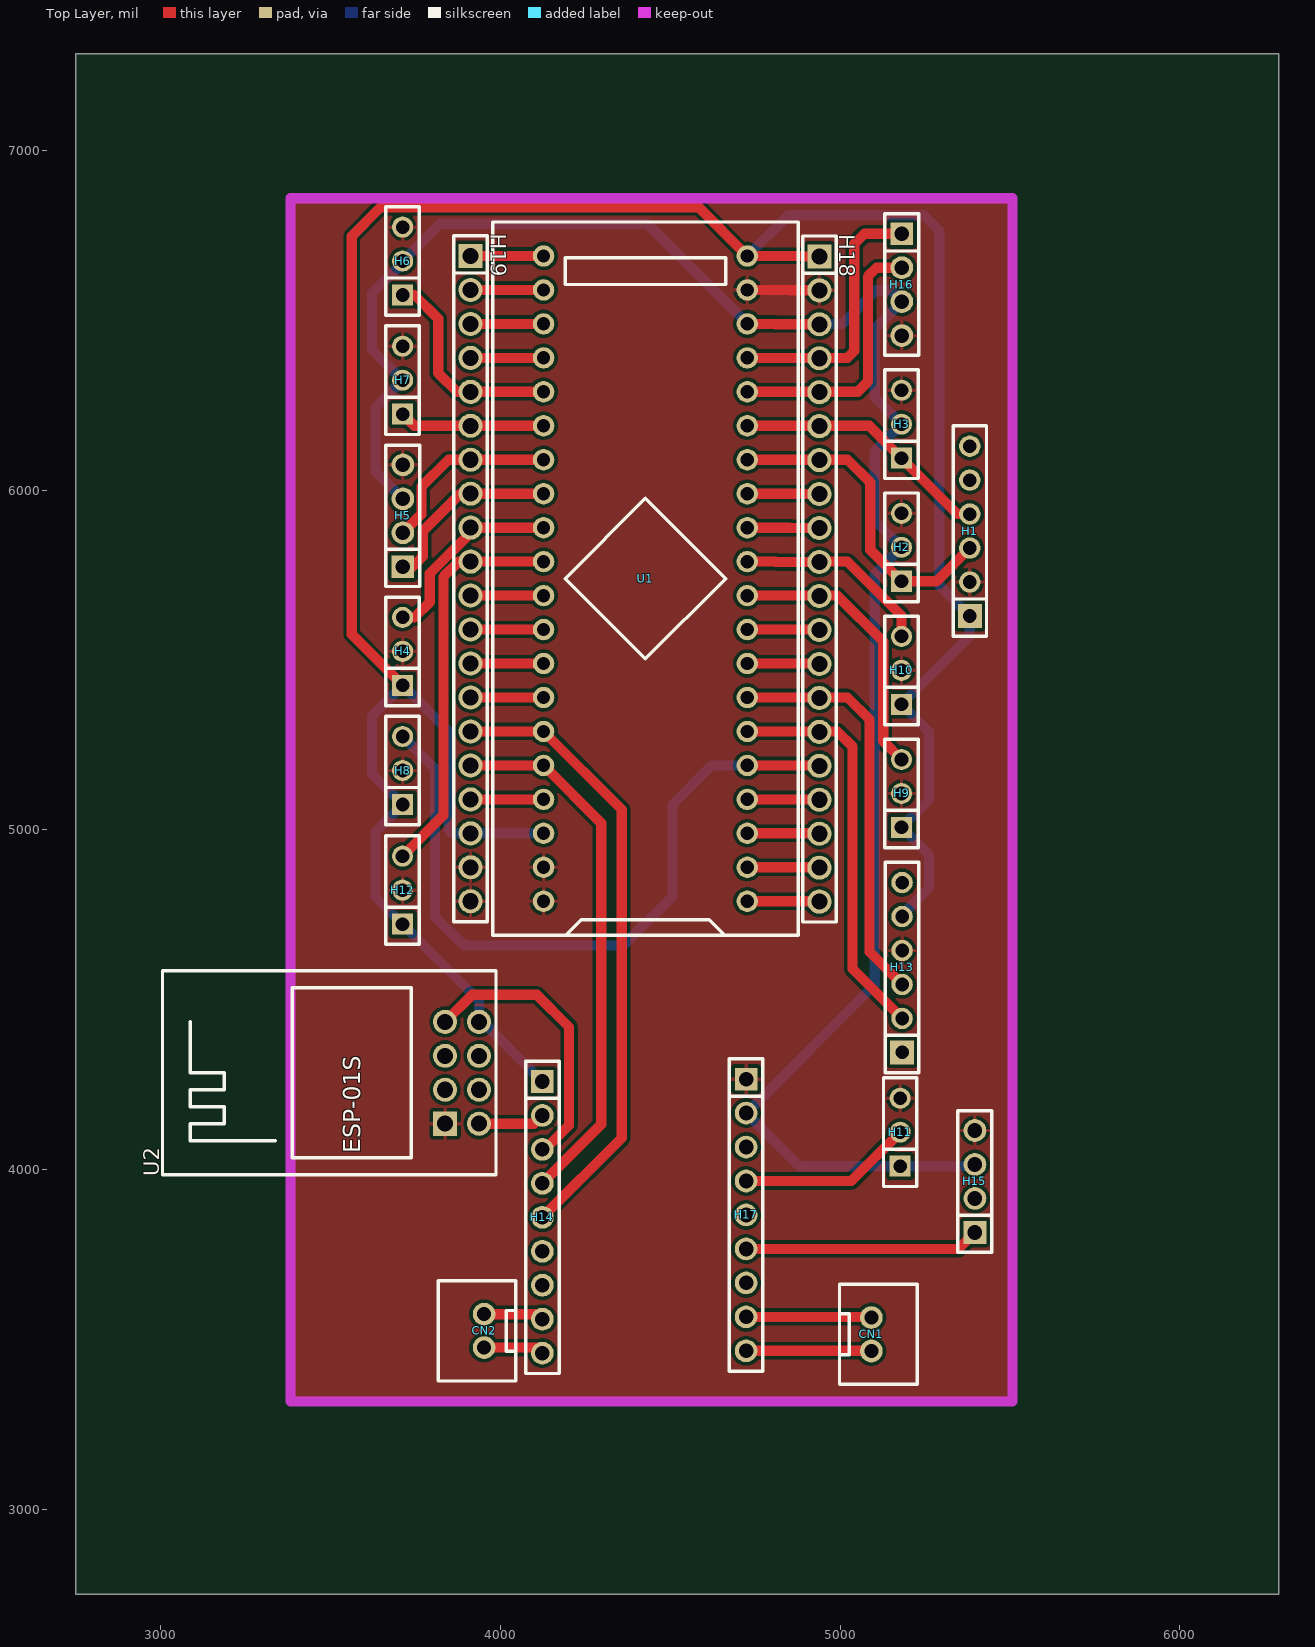
[diagram p0: Top Layer view]
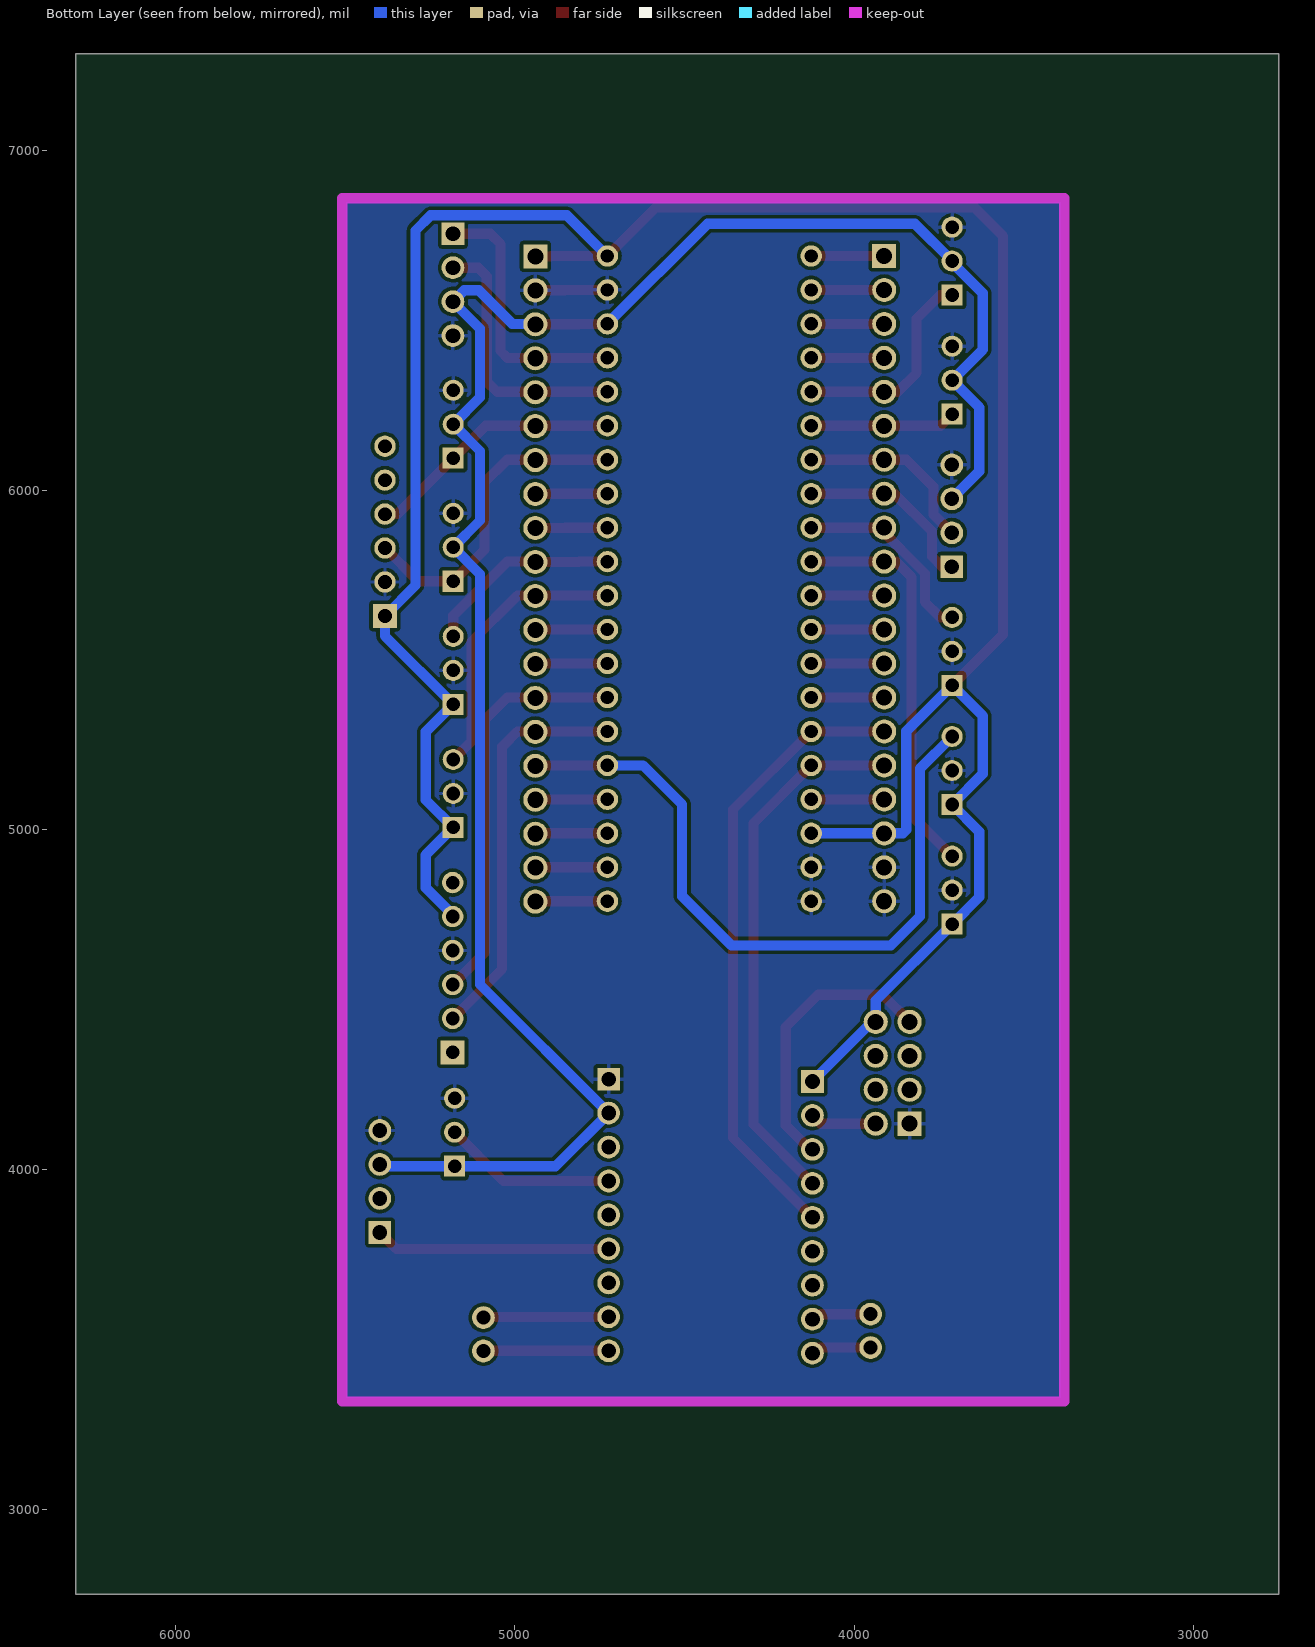
[diagram p1: Bottom Layer view, seen from below]
# Altium PCB MISC51613.pcbdoc
Units mil, origin at the board's own origin, x right, y up, seen from the top; angles counter-clockwise.
Board outline 3542 x 4535 mil, 2 copper layers (Top Layer, Bottom Layer), stack 62.206 mil thick; 23 components, 45 nets, 164 pads, 0 vias.

## Layer stack, top to bottom
Top Solder Mask Layer: solder mask 0.394, Dk 3.3
Top Layer: signal copper 1.379
Dielectric1: surface 59.449, FR4, Dk 4.5
Bottom Layer: signal copper 1.378
Bottom Solder Mask Layer: solder mask 0.394, Dk 3.3

## Board outline
6292,2750 2750,2750 2750,7285 6292,7285

## Design rules (kind name [scope] priority, off if disabled: settings)
BoardOutlineClearance copperThickness2oz_1 [All] p2 off: genericclearance=7.99 ignorepadtopadclearanceinfootprint=FALSE except(0: Arc-SplitContinuation Track-SplitContinuation SMDPad-SplitContinuation THPad-SplitContinuation Via-SplitContinuation Fill-SplitContinuation Region-SplitContinuation Poly-SplitContinuation Text-SplitContinuation Hole-SplitContinuation; 5.98: Arc-CutoutEdge Track-CutoutEdge SMDPad-CutoutEdge THPad-CutoutEdge Via-CutoutEdge Text-CutoutEdge; 6.9: Hole-OutlineEdge Hole-CutoutEdge; 10: Poly-OutlineEdge Poly-CutoutEdge; 11.81: Arc-OutlineEdge Track-OutlineEdge SMDPad-OutlineEdge THPad-OutlineEdge Via-OutlineEdge Fill-OutlineEdge Region-OutlineEdge Text-OutlineEdge Fill-CutoutEdge Region-CutoutEdge)
BoardOutlineClearance Plane_innerPlane_1 [All] p4 off: genericclearance=4.02 ignorepadtopadclearanceinfootprint=FALSE except(0: Arc-SplitContinuation Track-SplitContinuation SMDPad-SplitContinuation THPad-SplitContinuation Via-SplitContinuation Fill-SplitContinuation Region-SplitContinuation Poly-SplitContinuation Text-SplitContinuation Hole-SplitContinuation; 5.98: Arc-CutoutEdge Track-CutoutEdge SMDPad-CutoutEdge THPad-CutoutEdge Via-CutoutEdge Text-CutoutEdge; 6.9: Hole-OutlineEdge Hole-CutoutEdge; 10: Poly-OutlineEdge Poly-CutoutEdge; 11.81: Arc-OutlineEdge Track-OutlineEdge SMDPad-OutlineEdge THPad-OutlineEdge Via-OutlineEdge Fill-OutlineEdge Region-OutlineEdge Text-OutlineEdge Fill-CutoutEdge Region-CutoutEdge)
BoardOutlineClearance Copper_copperRegion_1 [All] p6 off: genericclearance=4.02 ignorepadtopadclearanceinfootprint=FALSE except(0: Arc-SplitContinuation Track-SplitContinuation SMDPad-SplitContinuation THPad-SplitContinuation Via-SplitContinuation Fill-SplitContinuation Region-SplitContinuation Poly-SplitContinuation Text-SplitContinuation Hole-SplitContinuation; 5.98: Arc-CutoutEdge Track-CutoutEdge SMDPad-CutoutEdge THPad-CutoutEdge Via-CutoutEdge Text-CutoutEdge; 6.9: Hole-OutlineEdge Hole-CutoutEdge; 10: Poly-OutlineEdge Poly-CutoutEdge; 11.81: Arc-OutlineEdge Track-OutlineEdge SMDPad-OutlineEdge THPad-OutlineEdge Via-OutlineEdge Fill-OutlineEdge Region-OutlineEdge Text-OutlineEdge Fill-CutoutEdge Region-CutoutEdge)
BoardOutlineClearance copperThickness1oz_1 [All] p8: genericclearance=4.02 ignorepadtopadclearanceinfootprint=FALSE except(0: Arc-SplitContinuation Track-SplitContinuation SMDPad-SplitContinuation THPad-SplitContinuation Via-SplitContinuation Fill-SplitContinuation Region-SplitContinuation Poly-SplitContinuation Text-SplitContinuation Hole-SplitContinuation; 5.98: Arc-CutoutEdge Track-CutoutEdge SMDPad-CutoutEdge THPad-CutoutEdge Via-CutoutEdge Text-CutoutEdge; 6.9: Hole-OutlineEdge Hole-CutoutEdge; 10: Poly-OutlineEdge Poly-CutoutEdge; 11.81: Arc-OutlineEdge Track-OutlineEdge SMDPad-OutlineEdge THPad-OutlineEdge Via-OutlineEdge Fill-OutlineEdge Region-OutlineEdge Text-OutlineEdge Fill-CutoutEdge Region-CutoutEdge)
Clearance copperThickness2oz [All] p1 off: gap=7.99 ignorepadtopadclearanceinfootprint=FALSE except(5.98: SMDPad-Track SMDPad-SMDPad THPad-Track SMDPad-THPad THPad-THPad Track-Via SMDPad-Via THPad-Via Via-Via Fill-SMDPad Region-SMDPad Fill-THPad Region-THPad Fill-Via Region-Via Fill-Fill Fill-Region Region-Region Arc-Track Arc-SMDPad Arc-THPad Arc-Via Fill-Arc Region-Arc Arc-Arc Text-Track SMDPad-Text Text-THPad Text-Via Fill-Text Region-Text Arc-Text Text-Text; 6.9: Hole-Track Hole-SMDPad Hole-THPad Hole-Via Fill-Hole Region-Hole Hole-Arc Hole-Text; 10: Poly-Track Poly-SMDPad Poly-THPad Poly-Via Poly-Fill Poly-Region Poly-Poly Poly-Arc Poly-Text Poly-Hole; 11.81: Fill-Track Region-Track)
Clearance Plane_innerPlane [All] p3 off: gap=4.02 ignorepadtopadclearanceinfootprint=FALSE except(5.98: SMDPad-Track SMDPad-SMDPad THPad-Track SMDPad-THPad THPad-THPad Track-Via SMDPad-Via THPad-Via Via-Via Fill-SMDPad Region-SMDPad Fill-THPad Region-THPad Fill-Via Region-Via Fill-Fill Fill-Region Region-Region Arc-Track Arc-SMDPad Arc-THPad Arc-Via Fill-Arc Region-Arc Arc-Arc Text-Track SMDPad-Text Text-THPad Text-Via Fill-Text Region-Text Arc-Text Text-Text; 6.9: Hole-Track Hole-SMDPad Hole-THPad Hole-Via Fill-Hole Region-Hole Hole-Arc Hole-Text; 10: Poly-Track Poly-SMDPad Poly-THPad Poly-Via Poly-Fill Poly-Region Poly-Poly Poly-Arc Poly-Text Poly-Hole; 11.81: Fill-Track Region-Track)
Clearance Copper_copperRegion [All] p5 off: gap=4.02 ignorepadtopadclearanceinfootprint=FALSE except(5.98: SMDPad-Track SMDPad-SMDPad THPad-Track SMDPad-THPad THPad-THPad Track-Via SMDPad-Via THPad-Via Via-Via Fill-SMDPad Region-SMDPad Fill-THPad Region-THPad Fill-Via Region-Via Fill-Fill Fill-Region Region-Region Arc-Track Arc-SMDPad Arc-THPad Arc-Via Fill-Arc Region-Arc Arc-Arc Text-Track SMDPad-Text Text-THPad Text-Via Fill-Text Region-Text Arc-Text Text-Text; 6.9: Hole-Track Hole-SMDPad Hole-THPad Hole-Via Fill-Hole Region-Hole Hole-Arc Hole-Text; 10: Poly-Track Poly-SMDPad Poly-THPad Poly-Via Poly-Fill Poly-Region Poly-Poly Poly-Arc Poly-Text Poly-Hole; 11.81: Fill-Track Region-Track)
Clearance copperThickness1oz [All] p7: gap=4.02 ignorepadtopadclearanceinfootprint=FALSE except(5.98: SMDPad-Track SMDPad-SMDPad THPad-Track SMDPad-THPad THPad-THPad Track-Via SMDPad-Via THPad-Via Via-Via Fill-SMDPad Region-SMDPad Fill-THPad Region-THPad Fill-Via Region-Via Fill-Fill Fill-Region Region-Region Arc-Track Arc-SMDPad Arc-THPad Arc-Via Fill-Arc Region-Arc Arc-Arc Text-Track SMDPad-Text Text-THPad Text-Via Fill-Text Region-Text Arc-Text Text-Text; 6.9: Hole-Track Hole-SMDPad Hole-THPad Hole-Via Fill-Hole Region-Hole Hole-Arc Hole-Text; 10: Poly-Track Poly-SMDPad Poly-THPad Poly-Via Poly-Fill Poly-Region Poly-Poly Poly-Arc Poly-Text Poly-Hole; 11.81: Fill-Track Region-Track)
DiffPairsRouting differentialPair [All] p1: maxlimit=6 minlimit=6 mostfreqgap=6 toplayer_minwidth=5 toplayer_prefwidth=10 toplayer_maxwidth=100 toplayer_mingap=6 toplayer_prefgap=6 toplayer_maxgap=6 bottomlayer_minwidth=5 bottomlayer_prefwidth=10 bottomlayer_maxwidth=100 bottomlayer_mingap=6 bottomlayer_prefgap=6 bottomlayer_maxgap=6 maxuncoupledlength=10
HoleToHoleClearance otherClearance [All] p1: gap=11.81 allowstackedmicrovias=TRUE
Length netLength [All] p1: minlimit=0 maxlimit=0
PasteMaskExpansion pasteMaskExpansion [All] p1: expansion=0
PlaneConnect innerPlane [All] p1: planeconnectstyle=Relief reliefexpansion=20 reliefentries=4 reliefconductorwidth=10 reliefairgap=10
PolygonConnect copperRegion [(InNet('GND'))] p1: connectstyle=Relief reliefconductorwidth=10 reliefentries=4 polygonreliefangle="90 Angle" airgapwidth=10 via.connectstyle=Relief via.reliefconductorwidth=10 via.reliefentries=4 via.polygonreliefangle="90 Angle" via.airgapwidth=10
RoutingVias viaSize [All] p1: holewidth=12.01 width=24.02 viastyle="Through Hole" minholewidth=11.81 minwidth=19.68 maxholewidth=248.03 maxwidth=393.7
SolderMaskExpansion solderMaskExpansion [IsVia] p1: expansion=-1000 istentingtop=TRUE
SolderMaskExpansion solderMaskExpansion [All] p2: expansion=2 istentingtop=FALSE
Width copperThickness2oz_2 [All] p1 off: maxlimit=100 minlimit=8 preferedwidth=10
Width copperThickness1oz_2 [All] p2: maxlimit=100 minlimit=5 preferedwidth=10

## Components (designator, comment, footprint, x,y, rotation, side; value= is the part's Value field where it differs from the comment)
CN1 "XH2.54*2P_through-hole" CONN-TH_2P-P2.50-XH2.54-2P 5092,3515 r90 top
CN2 "XH2.54*2P_through-hole" CONN-TH_2P-P2.50-XH2.54-2P 3952,3525 r270 top
H1 "" HDR-TH_6P-P2.54-V-F 5382,5880 r90 top
H2 "" HDR-TH_3P-P2.54-V-F 5181.06,5832.25 r90 top
H3 "" HDR-TH_3P-P2.54-V-F 5181.06,6194.66 r90 top
H4 "" HDR-TH_3P-P2.54-V-F 3712,5525.79 r90 top
H5 "" HDR-TH_4P-P2.54-V-F 3712.79,5925 r90 top
H6 "" HDR-TH_3P-P2.54-V-F 3712,6675 r90 top
H7 "" HDR-TH_3P-P2.54-V-F 3712,6324.21 r90 top
H8 "" HDR-TH_3P-P2.54-V-F 3712,5175 r90 top
H9 "" HDR-TH_3P-P2.54-V-F 5181.06,5107.42 r90 top
H10 "" HDR-TH_3P-P2.54-V-F 5181.06,5469.83 r90 top
H11 "" HDR-TH_3P-P2.54-V-F 5177,4110 r90 top
H12 "" HDR-TH_3P-P2.54-V-F 3711.84,4822.79 r90 top
H13 "" HDR-TH_6P-P2.54-V-F 5182.63,4595 r90 top
H14 "" HDR-TH_9P-P2.54-V-F-1 4123.42,3859.44 r270 top
H15 "" HDR-TH_4P-P2.54-V-F 5397,3965 r90 top
H16 "" HDR-TH_4P-P2.54-V-F 5181.84,6605.51 r270 top
H17 "" HDR-TH_9P-P2.54-V-F-1 4723.42,3866.33 r270 top
H18 "" HDR-TH_20P-P2.54-V-F 4939.11,5738.84 r270 top
H19 "" HDR-TH_20P-P2.54-V-F 3912,5740 r270 top
U1 "STM32F103C8T6-Card" CONN-TH_L53.3-W22.9_STM32F103C8T6-CARD 4427,5740 r90 top
U2 "ESP-01S" WIFIM-TH_ESP-01S 3887,4285 r90 top

## Footprints (in the part's own frame and the unit in brackets; to place one, negate y for a bottom-side part, rotate by r counter-clockwise, add the part's x,y. Pads: shape width x height; smd on the part's side, far side on the other; paste and mask are expansions set on the pad)
CONN-TH_2P-P2.50-XH2.54-2P [mm]
  round 1.7 hole 1.05 paste+0 mask+0.05: 1(1.25,0) 2(-1.25,0)
  silkscreen extent -3.75,-3.42 3.75,2.37
CONN-TH_L53.3-W22.9_STM32F103C8T6-CARD [mm]
  round 1.6 hole 1: 1(-24.13,-7.62) 2(-21.59,-7.62) 3(-19.05,-7.62) 4(-16.51,-7.62) 5(-13.97,-7.62) 6(-11.43,-7.62) 7(-8.89,-7.62) 8(-6.35,-7.62) 9(-3.81,-7.62) 10(-1.27,-7.62) 11(1.27,-7.62) 12(3.81,-7.62) 13(6.35,-7.62) 14(8.89,-7.62) 15(11.43,-7.62) 16(13.97,-7.62) 17(16.51,-7.62) 18(19.05,-7.62) 19(21.59,-7.62) 20(24.13,-7.62) 21(24.13,7.62) 22(21.59,7.62) 23(19.05,7.62) 24(16.51,7.62) 25(13.97,7.62) 26(11.43,7.62) 27(8.89,7.62) 28(6.35,7.62) 29(3.81,7.62) 30(1.27,7.62) 31(-1.27,7.62) 32(-3.81,7.62) 33(-6.35,7.62) 34(-8.89,7.62) 35(-11.43,7.62) 36(-13.97,7.62) 37(-16.51,7.62) 38(-19.05,7.62) 39(-21.59,7.62) 40(-24.13,7.62)
  silkscreen extent -26.67,-11.43 26.67,11.43
HDR-TH_3P-P2.54-V-F [mil]
  rect 62x62 hole 40.16: 1(-100,0)
  round 62 hole 40.16: 2(0,0) 3(100,0)
  silkscreen extent -160,-49 160,49
HDR-TH_4P-P2.54-V-F [mm]
  rect 1.7x1.7 hole 1.1: 1(-3.81,0)
  round 1.7 hole 1.1: 2(-1.27,0) 3(1.27,0) 4(3.81,0)
  silkscreen extent -5.29,-1.27 5.29,1.27
HDR-TH_6P-P2.54-V-F [mm]
  rect 1.8x1.8 hole 1.02: 1(-6.35,0)
  round 1.6 hole 1.02: 2(-3.81,0) 3(-1.27,0) 4(1.27,0) 5(3.81,0) 6(6.35,0)
  silkscreen extent -7.87,-1.25 7.87,1.25
HDR-TH_9P-P2.54-V-F-1 [mm]
  rect 1.7x1.7 hole 1.1: 1(-10.16,0)
  round 1.7 hole 1.1: 2(-7.62,0) 3(-5.08,0) 4(-2.54,0) 5(0,0) 6(2.54,0) 7(5.08,0) 8(7.62,0) 9(10.16,0)
  silkscreen extent -11.68,-1.25 11.68,1.25
HDR-TH_20P-P2.54-V-F [mm]
  rect 1.8x1.8 hole 1.2: 1(-24.13,0)
  round 1.8 hole 1.2: 2(-21.59,0) 3(-19.05,0) 4(-16.51,0) 5(-13.97,0) 6(-11.43,0) 7(-8.89,0) 8(-6.35,0) 9(-3.81,0) 10(-1.27,0) 11(1.27,0) 12(3.81,0) 13(6.35,0) 14(8.89,0) 15(11.43,0) 16(13.97,0) 17(16.51,0) 18(19.05,0) 19(21.59,0) 20(24.13,0)
  silkscreen extent -25.65,-1.25 25.65,1.25
WIFIM-TH_ESP-01S [mm]
  rect 1.8x1.8 hole 1.2: 1(-3.81,1.27)
  round 1.8 hole 1.2: 2(-1.27,1.27) 3(1.27,1.27) 4(3.81,1.27) 5(3.81,-1.27) 6(1.27,-1.27) 7(-1.27,-1.27) 8(-3.81,-1.27)
  silkscreen extent -7.62,-2.54 7.62,22.4

## Nets (pads, with @x,y where several pads share a name; then routed paths per layer and width w, separated by ;. In a path a pad name is that pad's centre, name@x,y a point inside that pad or via, vN(x,y) a via of type N, cw(c..) or ccw(c..) an arc to the next point about the centre after c; other vN are vias at no path point)
$1N17166: H15.1 H17.6 | length 693.7
  Top Layer w30: H17.6 5348.33,3766.33 H15.1
$1N17173: H11.2 H17.4 | length 513.1
  Top Layer w30: H17.4 5033.33,3966.33 H11.2
+5V: H2.2 H3.2 H5.3 H6.2 H7.2 H11.1 H15.3 H16.3 H17.2 H18.3 U1.18 | length 5984.5
  Top Layer w30: U1.18 4809.67,6490 4810.83,6488.84 H18.3
  Bottom Layer w30: H5.3 3632,6055.79 3632,6244.21 H7.2 3622,6414.21 3622,6580 3712,6670 H6.2 3822,6785 4432,6785 U1.18 ; H18.3@4939.11,6490 5007,6490 5105.96,6588.96 5148.39,6588.96 H16.3 5102,6475.66 5102,6273.72 H3.2 5102,6115.61 5102,5911.3 H2.2 5102,5753.19 5102,4544.92 H17.2 4879.75,4010 H11.1 5392,4010 H15.3
GND: H1.2 H2.3 H3.3 H4.2 H5.4 H6.3 H7.3 H8.2 H9.2 H10.2 H11.3 H12.2 H13.4 H15.4 H16.4 H17.1 H18.2 H19.19 H19.20 U1.19 U1.39 U1.40 U2.1 | length 212.6
  Top Layer w30: U1.19 4851.09,6590 4852.25,6588.84 H18.2
MIC+: CN1.1 H17.8 | length 369.5
  Top Layer w30: H17.8 5089.88,3566.33 CN1.1
MIC-: CN1.2 H17.9 | length 368.8
  Top Layer w30: H17.9 5091.45,3466.33 CN1.2
NRST: H19.17 U1.37 | length 215
  Top Layer w30: H19.17 U1.37
PA0: H6.1 H19.5 U1.25 | length 626.8
  Top Layer w30: H6.1 3747,6575 3817,6505 3817,6345 3872,6290 H19.5 U1.25
PA1: H7.1 H19.6 U1.26 | length 429.2
  Top Layer w30: H7.1 3746.21,6190 H19.6 U1.26
PA2: H5.2 H19.7 U1.27 | length 550.6
  Top Layer w30: H5.2 3767.24,5929.45 3767.24,6010.24 3847,6090 H19.7 U1.27
PA3: H5.1 H19.8 U1.28 | length 546.8
  Top Layer w30: H5.1 3741.25,5775 3771.25,5805 3771.25,5879.25 3882,5990 U1.28
PA4: H4.3 H19.9 U1.29 | length 573.8
  Top Layer w30: H4.3 3747,5625.79 3792,5670.79 3792,5755 3927,5890 U1.29
PA5: H12.3 H19.10 U1.30 | length 1185.6
  Top Layer w30: H12.3 3832,5042.94 3832,5745 3877,5790 U1.30
PA6: H19.11 U1.31 | length 215
  Top Layer w30: H19.11 U1.31
PA7: H19.12 U1.32 | length 215
  Top Layer w30: H19.12 U1.32
PA8: H8.3 H18.16 U1.5 | length 2114.8
  Top Layer w30: U1.5 4937.94,5190 H18.16
  Bottom Layer w30: H8.3 3807,5180 3807,4745 3892,4660 4362,4660 4507,4805 4507,5075 4622,5190 U1.5
PA9: H13.2 H18.15 U1.6 | length 1189
  Top Layer w30: U1.6 4992,5290 5037,5245 5037,4590.63 H13.2
PA10: H13.3 H18.14 U1.7 | length 1206.5
  Top Layer w30: U1.7 5022,5390 5087,5325 5087,4640.63 H13.3
PA11: H18.13 U1.8 | length 212.6
  Top Layer w30: U1.8 4937.94,5490 H18.13
PA12: H18.12 U1.9 | length 212.6
  Top Layer w30: U1.9 4937.94,5590 H18.12
PA15: H9.3 H18.11 U1.10 | length 827.5
  Top Layer w30: U1.10 H18.11@4937.94,5690 ; H18.11 H18.11@4937.94,5690 ; H9.3 5127,5261.47 5127,5555 4992,5690 H18.11@4937.94,5690
PB0: H19.13 U1.33 | length 215
  Top Layer w30: H19.13 U1.33
PB1: H19.14 U1.34 | length 215
  Top Layer w30: H19.14 U1.34
PB3: H10.3 H18.10 U1.11 | length 581.5
  Top Layer w30: U1.11 4809.67,5790 4810.83,5788.84 H18.10 ; H18.10@4939.11,5790 5022,5790 5181.06,5630.94 H10.3
PB4: H18.9 U1.12 | length 212.6
  Top Layer w30: U1.12 4851.09,5890 4852.25,5888.84 H18.9
PB5: H18.8 U1.13 | length 212.6
  Top Layer w30: U1.13 4892.51,5990 4893.67,5988.84 H18.8
PB6: H1.3 H2.1 H18.7 U1.14 | length 960.1
  Top Layer w30: U1.14 5022,6090 5088.71,6023.29 5088.71,5824.6 H2.1 5284.25,5732.25 H1.3
PB7: H1.4 H3.1 H18.6 U1.15 | length 762.7
  Top Layer w30: U1.15 5085.72,6190 H3.1 5345.72,5930 H1.4
PB8: H16.2 H18.5 U1.16 | length 787.8
  Top Layer w30: U1.16 5052,6290 5082,6320 5082,6630 5107.51,6655.51 H16.2
PB9: H16.1 H18.4 U1.17 | length 791.1
  Top Layer w30: U1.17 5022,6390 5042,6410 5042,6725.51 5072,6755.51 H16.1
PB10: H14.5 H19.15 U1.35 | length 1837.6
  Top Layer w30: H19.15 U1.35 4357,5060 4357,4093.03 H14.5
PB11: H14.4 H19.16 U1.36 | length 1587.9
  Top Layer w30: H19.16 U1.36 4297,5020 4297,4133.03 H14.4
PB12: H18.20 U1.1 | length 212.6
  Top Layer w30: U1.1 4937.94,4790 H18.20
PB13: H18.19 U1.2 | length 212.6
  Top Layer w30: U1.2 4937.94,4890 H18.19
PB14: H18.18 U1.3 | length 212.6
  Top Layer w30: U1.3 4937.94,4990 H18.18
PB15: H18.17 U1.4 | length 212.6
  Top Layer w30: U1.4 4937.94,5090 H18.17
PC13: H19.2 U1.22 | length 215
  Top Layer w30: H19.2 U1.22
PC14: H19.3 U1.23 | length 215
  Top Layer w30: H19.3 U1.23
PC15: H19.4 U1.24 | length 215
  Top Layer w30: H19.4 U1.24
RX: H14.3 U2.4 | length 835.3
  Top Layer w30: U2.4 3917,4515 4107,4515 4202,4420 4202,4130 4131.44,4059.44 H14.3
SPK+: CN2.1 H14.9 | length 178.2
  Top Layer w30: CN2.1 4107.08,3475.78 H14.9
SPK-: CN2.2 H14.8 | length 177.5
  Top Layer w30: CN2.2 4108.65,3574.22 H14.8
TX: H14.2 U2.8 | length 196.5
  Top Layer w30: U2.8 4098.97,4135 H14.2
VBAT: H19.1 U1.21 | length 215
  Top Layer w30: H19.1 U1.21
VCC: H1.1 H4.1 H8.1 H9.1 H10.1 H12.1 H13.5 H14.1 H18.1 H19.18 U1.20 U1.38 U2.5 | length 8013.8
  Top Layer w30: H4.1 3562,5575.79 3562,6748.19 3647,6833.19 4583.81,6833.19 U1.20 4892.51,6690 4893.67,6688.84 H18.1
  Bottom Layer w30: H14.1 3947.86,4435 U2.5 3937,4497.63 H12.1 3632,4802.63 3632,4995 H8.1 3622,5165 3622,5335.79 H4.1 3847,5290.79 3847,5000 3857,4990 H19.18 U1.38 ; U1.20 4847,6810 5247,6810 5292,6765 5292,5720 H1.1 5382,5570.78 H10.1 5262,5288.89 5262,5088.36 H9.1 5262,4926.47 5262,4830 5182.63,4750.63 H13.5
pads on no net: H1.5 H1.6 H13.1 H13.6 H14.6 H14.7 H15.2 H17.3 H17.5 H17.7 U2.2 U2.3 U2.6 U2.7

## Polygon pours and split planes (outlines as drawn)
GND on Top Layer (solid, remove dead copper, pour order 0): 3152,7035 3152,3020 6042,3020 6042,7035
GND on Bottom Layer (solid, remove dead copper, pour order 2): 3252,7005 3252,3000 5757,3000 5757,7005

## Keep-outs
Board Outline Layer:
  lines w30: 3382,3316.69 3382,6860 5507.98,6860 5507.98,3316.69 3382,3316.69